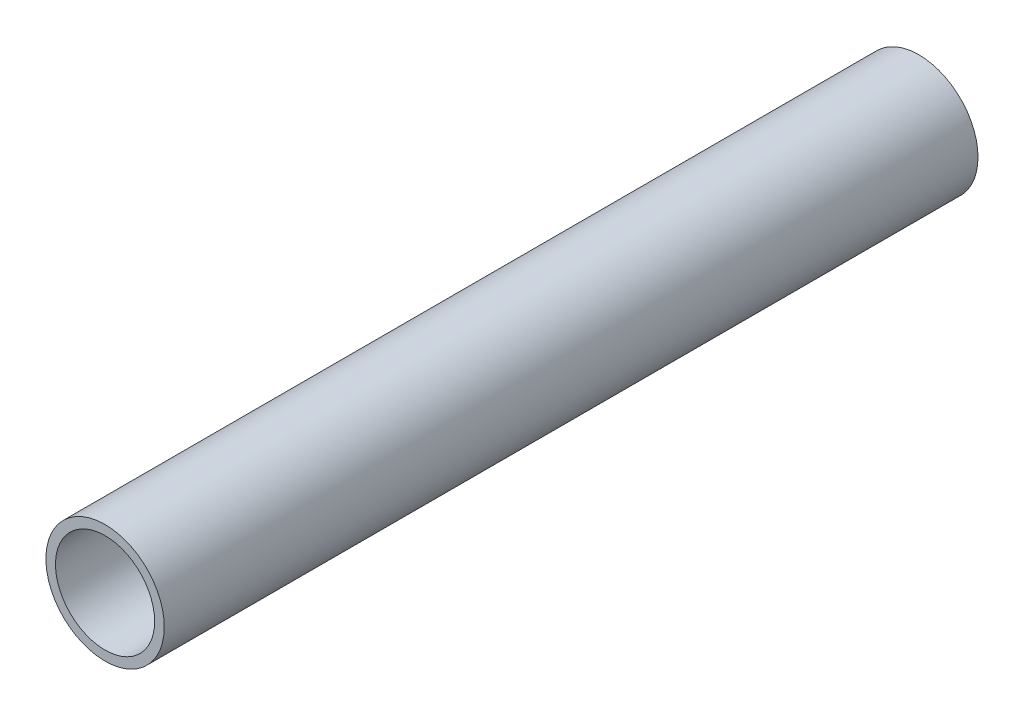
SolidWorks part; units mm, degrees
ref_plane "Front Plane" through (0, 0, 0) normal (0, 0, 1) x (1, 0, 0)
ref_plane "Top Plane" through (0, 0, 0) normal (0, 1, 0) x (1, 0, 0)
ref_plane "Right Plane" through (0, 0, 0) normal (1, 0, 0) x (0, 0, -1)
sketch "Sketch1" plane through (0, 0, 0) normal (0, 0, 1) x (1, 0, 0)
  circle A0 centre (0, 0) radius 40
  dimension "D1" = 80
extrude "Boss-Extrude1" add sketch "Sketch1" along normal blind 550
sketch "Sketch2" plane through (0, 0, 550) normal (0, 0, 1) x (1, 0, 0)
  circle A0 centre (0, 0) radius 33.5
  dimension "D1" = 67
extrude "Cut-Extrude1" cut sketch "Sketch2" against normal blind 90
